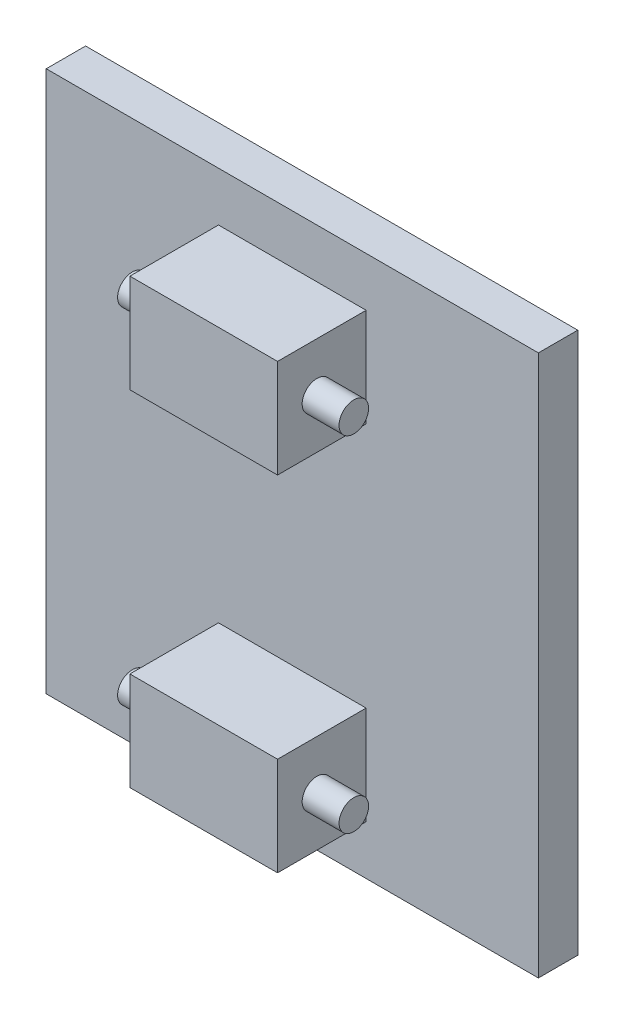
SolidWorks part; units mm, degrees
ref_plane "Front Plane" through (0, 0, 0) normal (0, 0, 1) x (1, 0, 0)
ref_plane "Top Plane" through (0, 0, 0) normal (0, 1, 0) x (1, 0, 0)
ref_plane "Right Plane" through (0, 0, 0) normal (1, 0, 0) x (0, 0, -1)
other "Configuration Table"
sketch "Sketch1" plane through (0, 0, 0) normal (0, 0, 1) x (1, 0, 0)
  line L1 (-50, 55) -> (50, 55)
  line L2 (-50, 55) -> (-50, -55)
  line L3 (-50, -55) -> (50, -55)
  line L4 (50, 55) -> (50, -55)
  line L5 (-50, 55) -> (50, -55) construction
  line L6 (-50, -55) -> (50, 55) construction
  point P0 (0, 0)
  dimension "D1" = 100
  dimension "D2" = 110
extrude "Boss-Extrude1" add sketch "Sketch1" along normal blind 8
sketch "Sketch2" plane through (0, 0, 8) normal (0, 0, 1) x (1, 0, 0)
  line L1 (-15, 25) -> (15, 25)
  line L2 (-15, 25) -> (-15, 45)
  line L3 (-15, 45) -> (15, 45)
  line L4 (15, 25) -> (15, 45)
  line L5 (-15, 25) -> (15, 45) construction
  line L6 (-15, 45) -> (15, 25) construction
  line L8 (-15, -25) -> (15, -25)
  line L9 (-15, -25) -> (-15, -45)
  line L10 (-15, -45) -> (15, -45)
  line L11 (15, -25) -> (15, -45)
  line L12 (-15, -25) -> (15, -45) construction
  line L13 (-15, -45) -> (15, -25) construction
  line L14 (-50, -55) -> (50, -55) construction
  line L15 (50, 55) -> (-50, 55) construction
  point P0 (0, 35)
  point P7 (0, -35)
  dimension "D1" = 30
  dimension "D2" = 30
  dimension "D3" = 20
  dimension "D4" = 20
  dimension "D5" = 10
  dimension "D6" = 10
extrude "Boss-Extrude2" add sketch "Sketch2" along normal blind 18
sketch "Sketch3" plane through (0, 0, 0) normal (1, 0, 0) x (0, 0, -1)
  line L0 (-26, 25) -> (-26, 45) construction
  circle A0 centre (-18, 35) radius 3
  circle A1 centre (-18, -35) radius 3
  dimension "D1" = 6
  dimension "D2" = 6
  dimension "D3" = 8
sketch "Sketch4" plane through (0, 0, 0) normal (0, 0, -1) x (-1, 0, 0)
  line L1 (-42.6492, 47.8173) -> (-13.3038, 47.8173)
  line L2 (-42.6492, 47.8173) -> (-42.6492, -43.7508)
  line L3 (-42.6492, -43.7508) -> (-13.3038, -43.7508)
  line L4 (-13.3038, 47.8173) -> (-13.3038, -43.7508)
  line L5 (-42.6492, 47.8173) -> (-13.3038, -43.7508) construction
  line L6 (-42.6492, -43.7508) -> (-13.3038, 47.8173) construction
  line L7 (11.3395, 47.8173) -> (44.0187, 47.8173)
  line L8 (11.3395, 47.8173) -> (11.3395, -44.2865)
  line L9 (11.3395, -44.2865) -> (44.0187, -44.2865)
  line L10 (44.0187, 47.8173) -> (44.0187, -44.2865)
  line L11 (11.3395, 47.8173) -> (44.0187, -44.2865) construction
  line L12 (11.3395, -44.2865) -> (44.0187, 47.8173) construction
  point P0 (-27.9765, 2.0333)
  point P5 (27.6791, 1.7654)
extrude "Cut-Extrude2" cut sketch "Sketch4" against normal blind 5
extrude "Boss-Extrude3" add sketch "Sketch3" along normal mid plane 45
